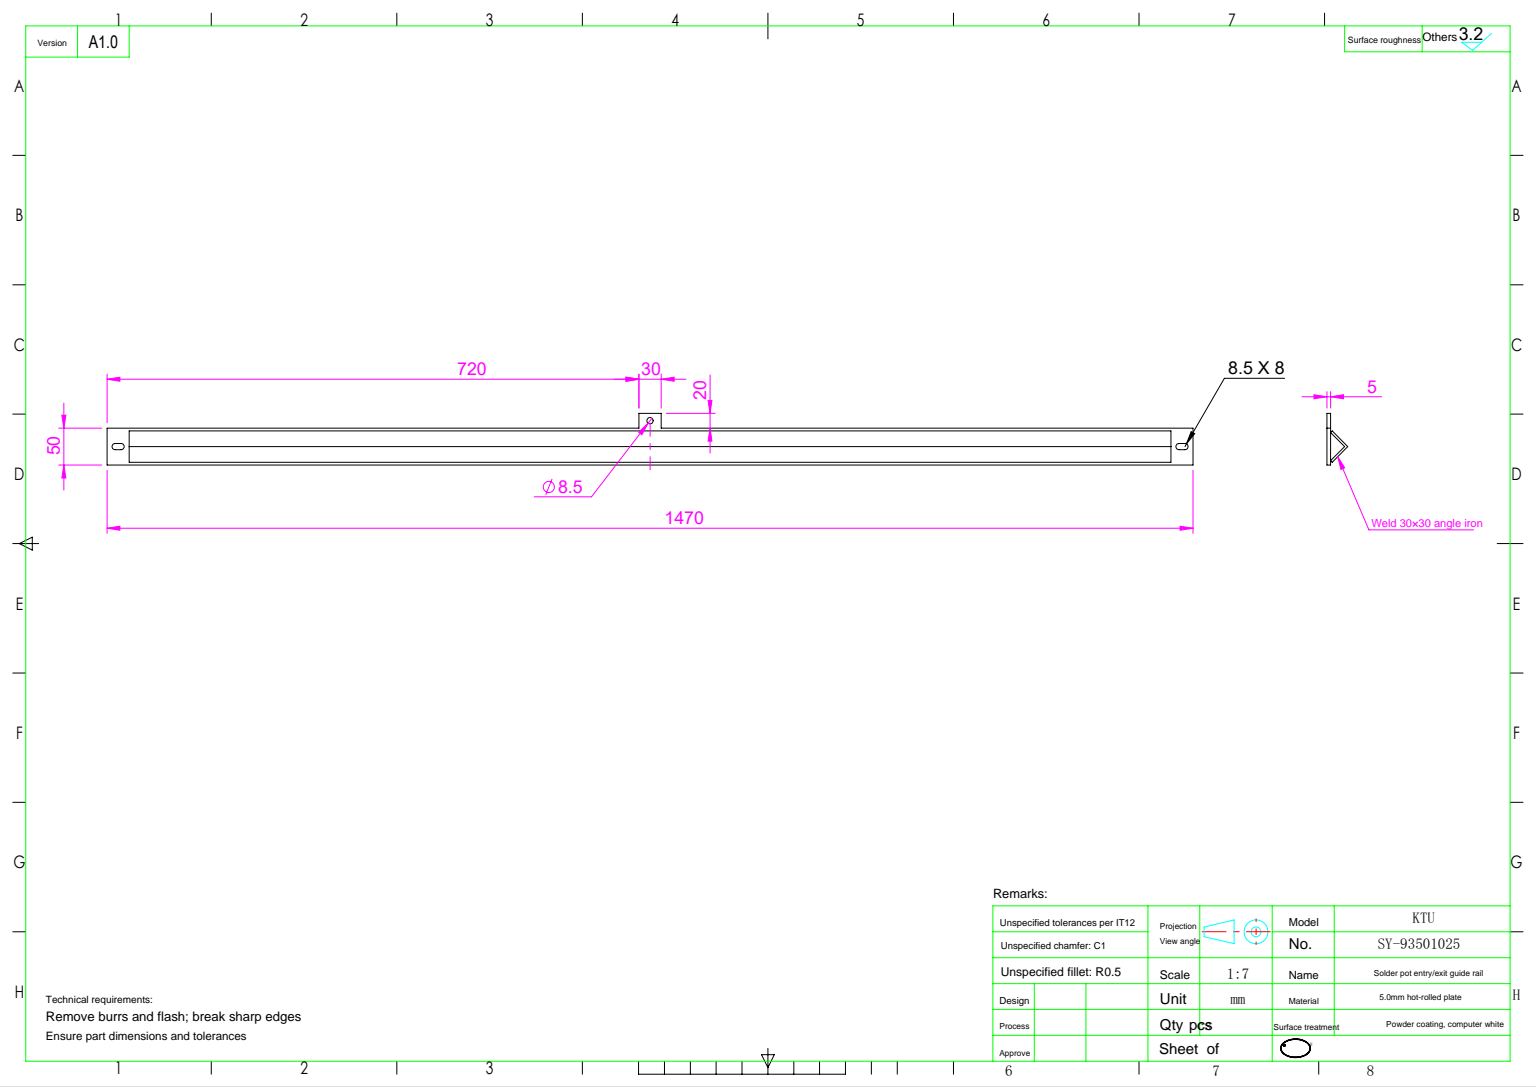
from build123d import *

# Parameters (mm, degrees)
SKETCH_1_W          = 1470
SKETCH_1_H          = 50
EXTRUDE_1_DEPTH     = 2.5
EXTRUDE_2_DEPTH     = 1410
CUT_EXTRUDE_1_DEPTH = 5
SKETCH_5_W          = 30
SKETCH_5_H          = 20
EXTRUDE_3_DEPTH     = 5
SKETCH_6_R          = 4.25
CUT_EXTRUDE_2_DEPTH = 5


with BuildPart() as part:
    # 草图1 → 凸台-拉伸1 (new, symmetric)
    with BuildSketch(Plane.XY):
        Rectangle(SKETCH_1_W, SKETCH_1_H)
    extrude(amount=EXTRUDE_1_DEPTH, both=True)

    # 草图4 → 切除-拉伸1 (cut)
    with BuildSketch(Plane.XY.offset(2.5)):
        with BuildLine():
            Line((716, 4.25), (724, 4.25))
            ThreePointArc((724, 4.25), (728.25, 0), (724, -4.25))
            Line((724, -4.25), (716, -4.25))
            ThreePointArc((716, -4.25), (711.75, 0), (716, 4.25))
        make_face()
        with BuildLine():
            Line((-716, -4.25), (-724, -4.25))
            ThreePointArc((-724, -4.25), (-728.25, 0), (-724, 4.25))
            Line((-724, 4.25), (-716, 4.25))
            ThreePointArc((-716, 4.25), (-711.75, 0), (-716, -4.25))
        make_face()
    extrude(amount=-CUT_EXTRUDE_1_DEPTH, mode=Mode.SUBTRACT)

    # 草图5 → 凸台-拉伸3 (add)
    with BuildSketch(Plane.XY.offset(2.5)):
        with Locations((0, 35)):
            Rectangle(SKETCH_5_W, SKETCH_5_H)
    extrude(amount=-EXTRUDE_3_DEPTH)

    # 草图6 → 切除-拉伸2 (cut)
    with BuildSketch(Plane.XY.offset(2.5)):
        with Locations((0, 35)):
            Circle(SKETCH_6_R)
    extrude(amount=-CUT_EXTRUDE_2_DEPTH, mode=Mode.SUBTRACT)


with BuildPart() as body_2:
    # 草图3 → 凸台-拉伸2 (new body)
    with BuildSketch(Plane.ZY.offset(705)):
        Polygon((2.5, 19.091883092), (21.591883092, 0), (2.5, -19.091883092), (4.621320344, -21.213203436), (25.834523779, 0), (4.621320344, 21.213203436), align=None)
    extrude(amount=-EXTRUDE_2_DEPTH)


solid = Compound([part.part, body_2.part])
